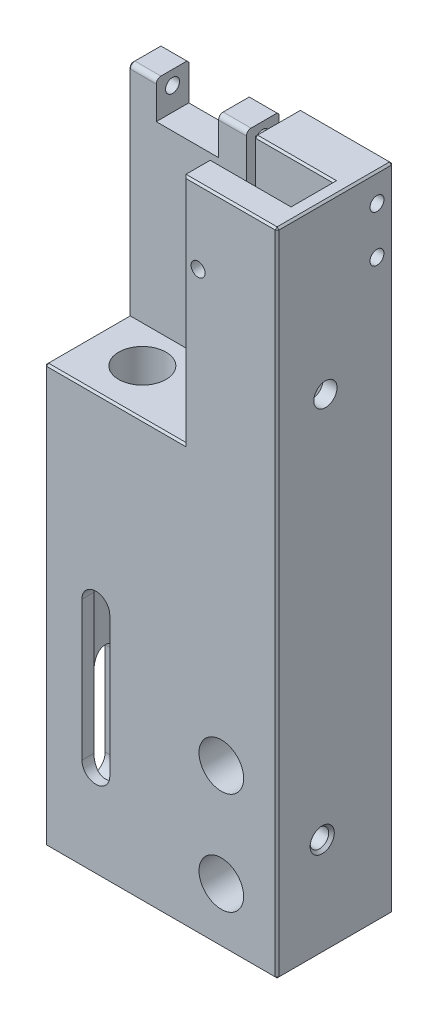
SolidWorks part; units mm, degrees
ref_plane "Front Plane" through (0, 0, 0) normal (0, 0, 1) x (1, 0, 0)
ref_plane "Top Plane" through (0, 0, 0) normal (0, 1, 0) x (1, 0, 0)
ref_plane "Right Plane" through (0, 0, 0) normal (1, 0, 0) x (0, 0, -1)
sketch "Sketch1" plane through (0, 0, 0) normal (0, 0, 1) x (1, 0, 0)
  line L1 (-12.5, 35) -> (12.5, 35)
  line L2 (-12.5, 35) -> (-12.5, -35)
  line L3 (-12.5, -35) -> (12.5, -35)
  line L4 (12.5, 35) -> (12.5, -35)
  line L5 (-12.5, 35) -> (12.5, -35) construction
  line L6 (-12.5, -35) -> (12.5, 35) construction
  point P0 (0, 0)
  dimension "D1" = 25
  dimension "D2" = 70
extrude "Boss-Extrude1" add sketch "Sketch1" along normal mid plane 12.5
sketch "Sketch2" plane through (0, -35, 0) normal (0, -1, 0) x (1, 0, 0)
  line L0 (-12.5, 6.25) -> (-12.5, -6.25) construction
  line L1 (-12.5, 6.25) -> (12.5, 6.25) construction
  circle A0 centre (-7, 1.25) radius 4
  dimension "D1" = 8
  dimension "D2" = 5.5
  dimension "D3" = 5
extrude "Cut-Extrude1" cut sketch "Sketch2" against normal blind 35
sketch "Sketch3" plane through (0, 0, 0) normal (0, -1, 0) x (1, 0, 0)
  circle A0 centre (-7, 1.25) radius 2.55
  dimension "D1" = 5.1
extrude "Cut-Extrude2" cut sketch "Sketch3" against normal through all
sketch "Sketch5" plane through (-12.5, 0, 0) normal (-1, 0, 0) x (0, 0, 1)
  line L1 (6.25, 35) -> (-2.75, 35)
  line L2 (6.25, 35) -> (6.25, 10)
  line L3 (6.25, 10) -> (-2.75, 10)
  line L4 (-2.75, 35) -> (-2.75, 10)
  dimension "D1" = 9
  dimension "D2" = 25
extrude "Cut-Extrude3" cut sketch "Sketch5" against normal blind 15
sketch "Sketch6" plane through (0, 0, 6.25) normal (0, 0, 1) x (1, 0, 0)
  line L0 (-7, 0) -> (-7, -24.9473) construction
  line L1 (-9.55, 0) -> (-4.45, 0) construction
  line L2 (-7, -10) -> (-7, -25) construction
  line L3 (-5.5, -10) -> (-5.5, -25)
  line L4 (-8.5, -10) -> (-8.5, -25)
  line L5 (-12.5, -35) -> (12.5, -35) construction
  arc A0 (-5.5, -10) -> (-8.5, -10) centre (-7, -10) ccw
  arc A1 (-8.5, -25) -> (-5.5, -25) centre (-7, -25) ccw
  point P6 (-7, -17.5)
  dimension "D1" = 1.5
  dimension "D2" = 15
  dimension "D3" = 10
extrude "Cut-Extrude4" cut sketch "Sketch6" against normal blind 5
sketch "Sketch7" plane through (0, 0, -6.25) normal (0, 0, -1) x (-1, 0, 0)
  line L0 (12.5, -35) -> (-12.5, -35) construction
  line L1 (12.5, 35) -> (12.5, -35) construction
  circle A0 centre (7, -16.0778) radius 1.75
  dimension "D1" = 3.5
  dimension "D2" = 5.5
  dimension "19" = 18.9222
extrude "Cut-Extrude5" cut sketch "Sketch7" against normal blind 6
sketch "Sketch8" plane through (0, 0, -6.25) normal (0, 0, -1) x (-1, 0, 0)
  line L0 (12.5, -35) -> (-12.5, -35) construction
  line L1 (-12.5, -35) -> (-12.5, 35) construction
  point P0 (-6.5, -18)
  point P1 (-6.5, -29)
  dimension "D1" = 6
  dimension "D2" = 11
  dimension "D3" = 6
hole_wizard "Hole size (per hex socket screw type) 1" positions "3DSketch1" profile "Sketch9" counterbore size "M4" standard "GB" end condition through all
sketch3d "3DSketch1"
  point P0 (6.5, -29, -6.25)
  point P3 (6.5, -18, -6.25)
sketch "Sketch9" plane through (6.5, -29, -6.25) normal (1, 0, 0) x (0, 1, 0)
  line L0 (0, 0) -> (0, 12.5)
  line L1 (0, 12.5) -> (2.4, 12.5)
  line L3 (2.4, 12.5) -> (2.4, 4.6)
  line L4 (2.4, 4.6) -> (4, 4.6)
  line L5 (4, 4.6) -> (4, 0)
  line L7 (4, 0) -> (0, 0)
  line L11 (0, -6.35) -> (0, 107.95) construction
  dimension "通孔孔直径" = 4.8
  dimension "通孔孔深度" = 12.5
  dimension "柱形沉头孔直径" = 8
  dimension "柱形沉头孔深度" = 4.6
fillet "Fillet1" radius 0.5 1 edges at (-5, 35, -2.75)
sketch "Sketch10" plane through (0, 0, -2.75) normal (0, 0, 1) x (1, 0, 0)
  line L0 (-12.5, 35) -> (2.5, 35) construction
  line L1 (-9.5, 35) -> (-2.8, 35)
  line L2 (-9.5, 35) -> (-9.5, 29.5)
  line L3 (-9.5, 29.5) -> (-2.8, 29.5)
  line L4 (-2.8, 35) -> (-2.8, 29.5)
  line L5 (-12.5, 34.5) -> (-12.5, 10) construction
  line L6 (2.5, 34.5) -> (2.5, 10) construction
  line L8 (2.5, 35) -> (0.2, 35)
  line L9 (2.5, 35) -> (2.5, 29.5)
  line L10 (2.5, 29.5) -> (0.2, 29.5)
  line L11 (0.2, 35) -> (0.2, 29.5)
  dimension "D1" = 3
  dimension "D2" = 5.5
  dimension "D3" = 5.3
  dimension "D4" = 3
extrude "Cut-Extrude6" cut sketch "Sketch10" against normal through all
sketch "Sketch11" plane through (0, 0, -2.75) normal (0, 0, 1) x (1, 0, 0)
  line L0 (2.5, 29.5) -> (2.5, 10) construction
  line L1 (0.2, 29.5) -> (2.5, 29.5)
  line L2 (0.2, 29.5) -> (0.2, 24.5)
  line L3 (0.2, 24.5) -> (2.5, 24.5)
  line L4 (2.5, 29.5) -> (2.5, 24.5)
  dimension "D1" = 5
extrude "Cut-Extrude7" cut sketch "Sketch11" against normal blind 1.75
sketch "Sketch13" plane through (0, 0, -6.25) normal (0, 0, -1) x (-1, 0, 0)
  line L0 (12.5, 35) -> (12.5, -35) construction
  line L1 (-0.2, 35) -> (12.5, 35)
  line L2 (-0.2, 35) -> (-0.2, 33.5)
  line L3 (-0.2, 33.5) -> (12.5, 33.5)
  line L4 (12.5, 35) -> (12.5, 33.5)
  line L5 (9.5, 29.5) -> (2.8, 29.5) construction
  dimension "4" = 4
extrude "Cut-Extrude8" cut sketch "Sketch13" against normal through all
fillet "Fillet2" radius 0.5 2 edges at (-1.3, 33.5, -2.75) (-11, 33.5, -2.75)
sketch "Sketch14" plane through (-12.5, 0, 0) normal (-1, 0, 0) x (0, 0, 1)
  line L0 (-6.25, 33.5) -> (-6.25, -35) construction
  line L1 (-3.25, 33.5) -> (-6.25, 33.5) construction
  circle A0 centre (-4.5, 32) radius 0.75
  dimension "D1" = 1.5
  dimension "D2" = 1.75
  dimension "D3" = 1.5
extrude "Cut-Extrude9" cut sketch "Sketch14" against normal through all
sketch "Sketch15" plane through (0, 35, 0) normal (0, 1, 0) x (1, 0, 0)
  line L0 (2.5, 2.75) -> (2.5, -6.25) construction
  line L1 (2.5, 1.25) -> (11, 1.25)
  line L2 (2.5, 1.25) -> (2.5, -3.25)
  line L3 (2.5, -3.25) -> (11, -3.25)
  line L4 (11, 1.25) -> (11, -3.25)
  line L5 (12.5, -6.25) -> (2.5, -6.25) construction
  line L6 (12.5, -6.25) -> (12.5, 6.25) construction
  dimension "D1" = 3
  dimension "D2" = 4.5
  dimension "D3" = 1.5
extrude "Cut-Extrude10" cut sketch "Sketch15" against normal up to surface (25 mm away) up to face at (-5, 10, 1.75)
sketch "Sketch16" plane through (-12.5, 0, 0) normal (-1, 0, 0) x (0, 0, 1)
  line L0 (1.25, -29.5) -> (1.25, -19.5) construction
  line L1 (-0.25, -29.5) -> (-0.25, -19.5)
  line L2 (2.75, -29.5) -> (2.75, -19.5)
  line L3 (6.25, -35) -> (-6.25, -35) construction
  line L4 (6.25, 10) -> (6.25, -35) construction
  arc A0 (-0.25, -29.5) -> (2.75, -29.5) centre (1.25, -29.5) ccw
  arc A1 (2.75, -19.5) -> (-0.25, -19.5) centre (1.25, -19.5) ccw
  point P2 (1.25, -24.5)
  dimension "D1" = 1.5
  dimension "D2" = 5.5
  dimension "D3" = 5
  dimension "D4" = 10
extrude "Cut-Extrude11" cut sketch "Sketch16" against normal up to vertex
sketch "Sketch17" plane through (-12.5, 0, 0) normal (-1, 0, 0) x (0, 0, 1)
  line L0 (-6.25, 33.5) -> (-6.25, -35) construction
  line L1 (-2.75, 10) -> (-1.25, 10) construction
  circle A0 centre (-5.05, 15.2) radius 0.6
  circle A1 centre (-5.05, 12) radius 0.6
  circle A2 centre (-5.05, 7.5) radius 0.6
  dimension "D1" = 1.2
  dimension "D2" = 1.2
  dimension "D3" = 2.5
  dimension "D4" = 4.5
  dimension "D5" = 3.2
extrude "Cut-Extrude12" cut sketch "Sketch17" against normal blind 15
sketch "Sketch18" plane through (0, 0, 6.25) normal (0, 0, 1) x (1, 0, 0)
  line L0 (12.5, 35) -> (2.5, 35) construction
  line L1 (2.5, 10) -> (2.5, 35) construction
  circle A0 centre (4, 27) radius 0.75
  dimension "D1" = 1.5
  dimension "D2" = 8
  dimension "2" = 1.5
extrude "Cut-Extrude13" cut sketch "Sketch18" against normal through all
sketch "Sketch19" plane through (0, 0, -6.25) normal (0, 0, -1) x (-1, 0, 0)
  line L0 (-9.5, 23) -> (-7.5, 23) construction
  line L1 (-9.5, 25) -> (-7.5, 25)
  line L2 (-9.5, 21) -> (-7.5, 21)
  line L3 (-12.5, -35) -> (-12.5, 35) construction
  line L4 (-12.5, 35) -> (-2.5, 35) construction
  arc A0 (-9.5, 25) -> (-9.5, 21) centre (-9.5, 23) ccw
  arc A1 (-7.5, 21) -> (-7.5, 25) centre (-7.5, 23) ccw
  point P2 (-8.5, 23)
  dimension "D1" = 2
  dimension "D2" = 2
  dimension "D3" = 3
  dimension "D4" = 12
extrude "Cut-Extrude14" cut sketch "Sketch19" against normal blind 7
chamfer "Chamfer1" distance 0.2 angle 45 1 edges at (-8.75, -16.0778, -6.25)
sketch "Sketch20" plane through (12.5, 0, 0) normal (1, 0, 0) x (0, 0, -1)
  circle A0 centre (-1.3951, -24.3426) radius 1
  dimension "D1" = 2
extrude "Cut-Extrude15" cut sketch "Sketch20" against normal blind 19
chamfer "Chamfer2" distance 0.3 angle 45 1 edges at (12.5, -23.3426, 1.3951)
sketch "Sketch21" plane through (12.5, 0, 0) normal (1, 0, 0) x (0, 0, -1)
  line L0 (-6.25, -35) -> (-6.25, 35) construction
  line L1 (-6.25, 35) -> (6.25, 35) construction
  circle A0 centre (-1.05, 17) radius 1.25
  dimension "D1" = 2.5
  dimension "D2" = 5.2
  dimension "D3" = 18
extrude "Cut-Extrude16" cut sketch "Sketch21" against normal blind 19
sketch "Sketch22" plane through (12.5, 0, 0) normal (1, 0, 0) x (0, 0, -1)
  line L0 (4.5, 32) -> (4.5, 26.9939) construction
  circle A0 centre (4.5, 26.9939) radius 0.75
  circle A1 centre (4.5, 32) radius 0.75 construction
extrude "Cut-Extrude17" cut sketch "Sketch22" against normal up to surface (10 mm away) up to face at (2.5, 32.75, -4.5)
chamfer "Chamfer3" distance 0.2 angle 45 24 edges at (-12.5, -0.75, -6.25) (-11, 33.5, -6.25) (-1.3, 33.5, -6.25) (0, -35, 6.25) (-12.5, 21.5, -2.75) (-12.5, 33.5, -4.75) (-12.5, 33.3536, -2.8964) (6.75, 35, 3.25) (11, 35, 1) (6.75, 35, -1.25) (2.5, 22.5, -1.25) (2.5, 22.5, 3.25) (-12.5, -12.5, 6.25) (-5, 10, 6.25) (2.5, 22.5, 6.25) (-12.5, 10, 1.75) (12.5, 0, 6.25) (0, -35, -6.25) (7.5, 35, -6.25) (12.5, 0, -6.25) (12.5, -35, 0) (-12.5, -35, 0) (12.5, 35, 0) (7.5, 35, 6.25)
